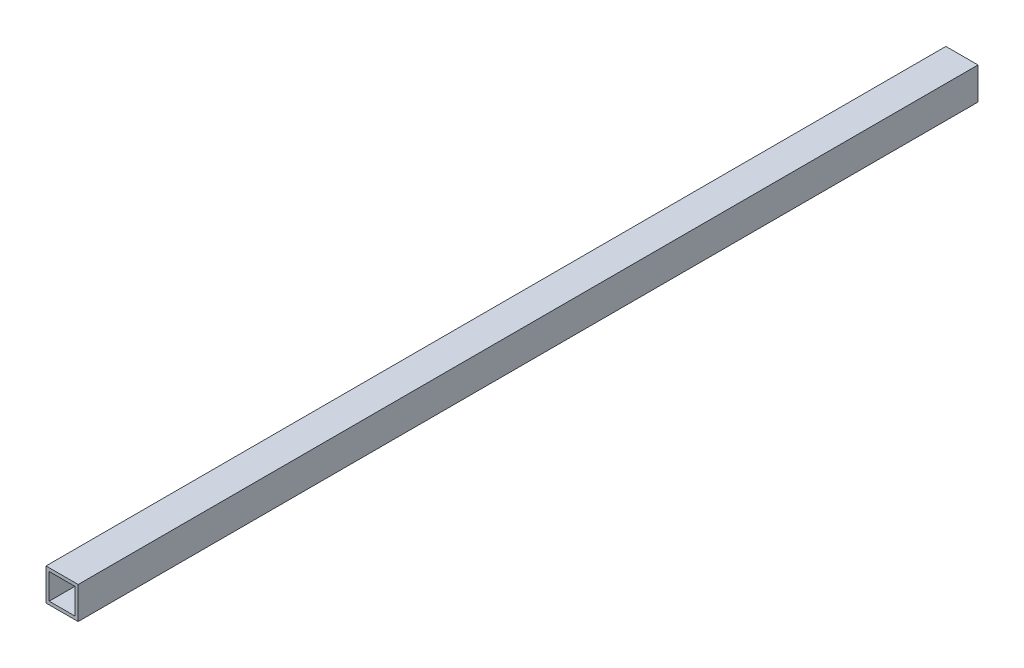
from build123d import *

# Parameters (mm, degrees)
SKETCH1_W           = 30
SKETCH1_H           = 30
BOSS_EXTRUDE1_DEPTH = 840
SKETCH2_W           = 24
SKETCH2_H           = 24
CUT_EXTRUDE1_DEPTH  = 840


with BuildPart() as part:
    # Sketch1 → Boss-Extrude1 (new body)
    with BuildSketch(Plane.XY):
        with Locations((3.8671875, 17.344389065)):
            Rectangle(SKETCH1_W, SKETCH1_H)
    extrude(amount=BOSS_EXTRUDE1_DEPTH)

    # Sketch2 → Cut-Extrude1 (cut)
    with BuildSketch(Plane.XY.offset(840)):
        with Locations((3.8671875, 17.344389065)):
            Rectangle(SKETCH2_W, SKETCH2_H)
    extrude(amount=-CUT_EXTRUDE1_DEPTH, mode=Mode.SUBTRACT)


solid = part.part
